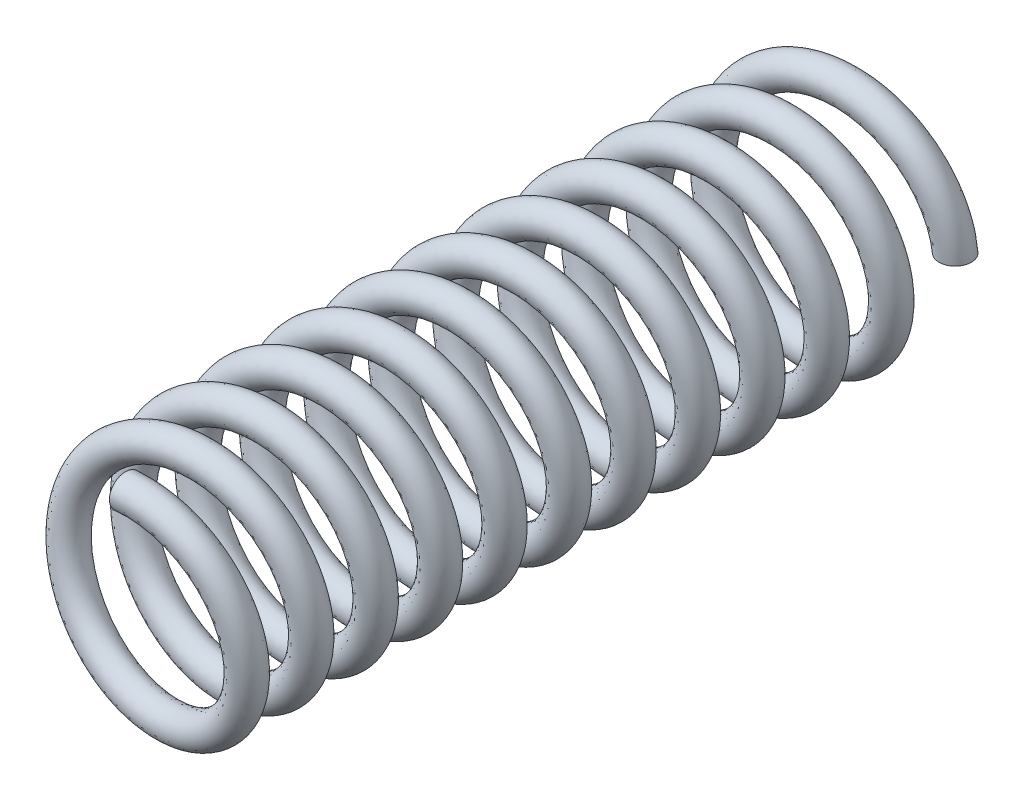
from build123d import *

# Parameters (mm, degrees)
SWEEP_1_PITCH  = 4
SWEEP_1_HEIGHT = 45
SWEEP_1_RADIUS = 6.5
SKETCH_2_R     = 1


with BuildPart() as part:
    # 扫描1: sweep along a helix
    with BuildLine() as sweep_1_path:
        Helix(SWEEP_1_PITCH, SWEEP_1_HEIGHT, SWEEP_1_RADIUS, center=(0, 0, 0), direction=(0, 0, 1))
    # 草图2 → 扫描1 (sweep)
    with BuildSketch(Plane(origin=(0, 0, 0), x_dir=(1, 0, 0), z_dir=(0, 1, 0))):
        with Locations((6.5, 0)):
            Circle(SKETCH_2_R)
    sweep(path=sweep_1_path.line, is_frenet=True)


solid = part.part
